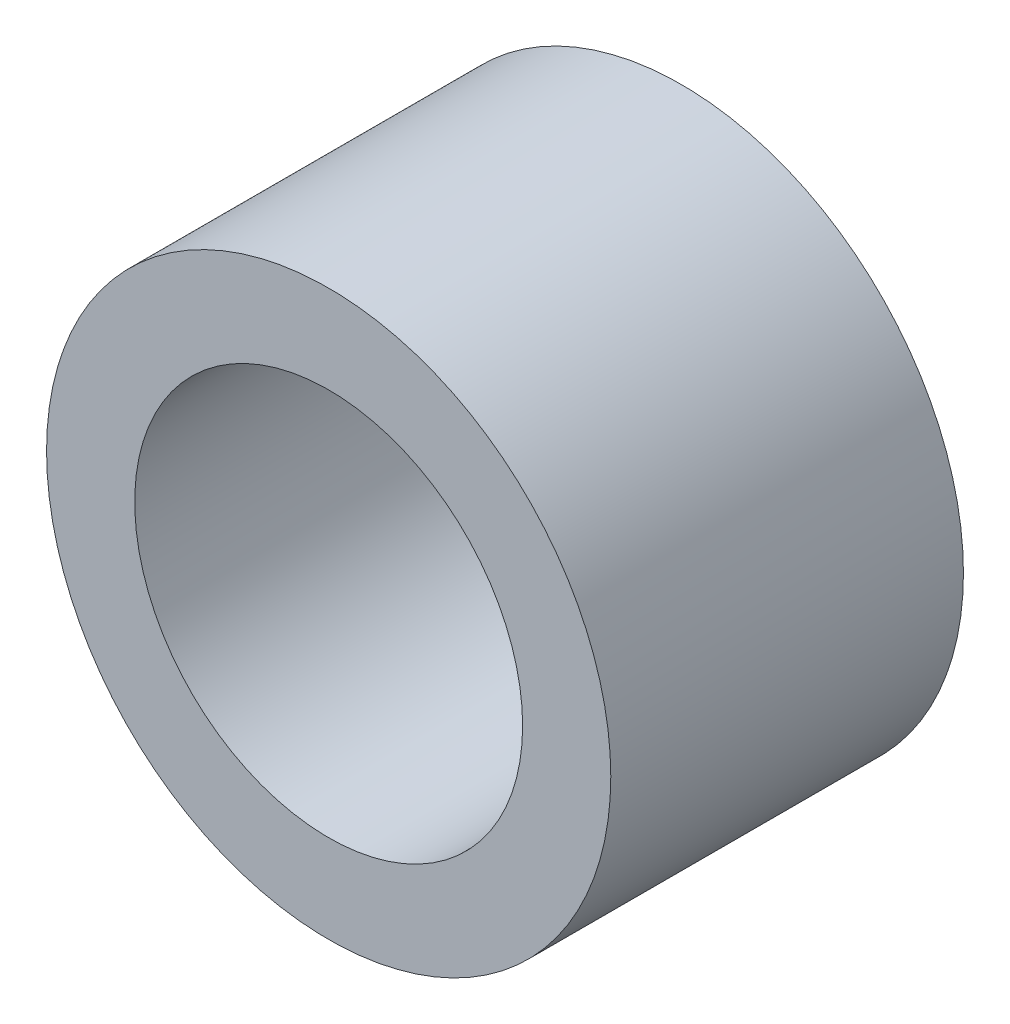
SolidWorks part; units mm, degrees
ref_plane "前视基准面" through (0, 0, 0) normal (0, 0, 1) x (1, 0, 0)
ref_plane "上视基准面" through (0, 0, 0) normal (0, 1, 0) x (1, 0, 0)
ref_plane "右视基准面" through (0, 0, 0) normal (1, 0, 0) x (0, 0, -1)
sketch "草图1" plane through (0, 0, 0) normal (0, 0, 1) x (1, 0, 0)
  circle A0 centre (0, 0) radius 8.25
  circle A1 centre (0, 0) radius 12
  dimension "D1" = 16.5
  dimension "D2" = 24
extrude "凸台-拉伸1" add sketch "草图1" along normal blind 15
